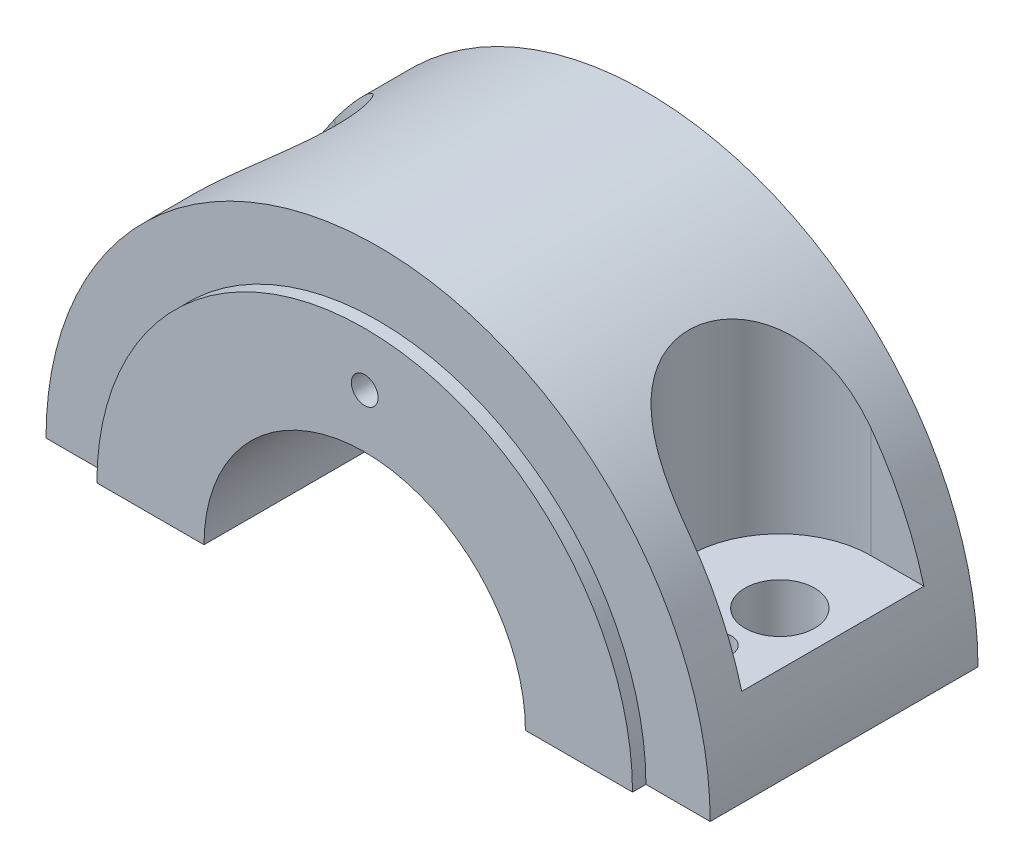
SolidWorks part; units mm, degrees
material "ZG270-500"
ref_plane "Front Plane" through (0, 0, 0) normal (0, 0, 1) x (1, 0, 0)
ref_plane "Top Plane" through (0, 0, 0) normal (0, 1, 0) x (1, 0, 0)
ref_plane "Right Plane" through (0, 0, 0) normal (1, 0, 0) x (0, 0, -1)
sketch "Sketch1" plane through (0, 0, 0) normal (0, 0, 1) x (1, 0, 0)
  line L0 (-62, 0) -> (-30, 0)
  line L1 (30, 0) -> (62, 0)
  arc A0 (62, 0) -> (-62, 0) centre (0, 0) ccw
  arc A1 (30, 0) -> (-30, 0) centre (0, 0) ccw
  dimension "D1" = 62
  dimension "D2" = 30
extrude "Boss-Extrude1" add sketch "Sketch1" along normal mid plane 50
sketch "Sketch2" plane through (0, 0, 0) normal (0, 0, 1) x (1, 0, 0)
  line L0 (-50, 0) -> (-30, 0)
  line L1 (30, 0) -> (50, 0)
  arc A0 (50, 0) -> (-50, 0) centre (0, 0) ccw
  arc A1 (30, 0) -> (-30, 0) centre (0, 0) ccw
  dimension "D1" = 50
  dimension "D2" = 30
extrude "Boss-Extrude2" add sketch "Sketch2" along normal mid plane 55
ref_plane "Plane1" through (0, 16, 0) normal (0, 1, 0) x (1, 0, 0)
sketch "Sketch3" plane through (0, 16, 0) normal (0, 1, 0) x (1, 0, 0)
  line L0 (-76.112, 0) -> (-75, 0) construction
  line L1 (0, 53.7818) -> (0, -41.5827) construction
  line L3 (-49.5568, 0) -> (74.644, 0) construction
  line L4 (-75, 17) -> (-50, 17)
  line L5 (-75, 17) -> (-75, -17)
  line L6 (-75, -17) -> (-50, -17)
  line L7 (75, -17) -> (50, -17)
  line L8 (75, 17) -> (75, -17)
  line L9 (75, 17) -> (50, 17)
  arc A0 (-50, -17) -> (-50, 17) centre (-50, 0) ccw
  arc A1 (50, -17) -> (50, 17) centre (50, 0) cw
  dimension "D1" = 17
  dimension "D2" = 100
  dimension "D3" = 34
  dimension "D4" = 150
extrude "Cut-Extrude1" cut sketch "Sketch3" along normal through all
sketch "Sketch4" plane through (0, 16, 0) normal (0, 1, 0) x (1, 0, 0)
  line L0 (-82.8581, 0) -> (79.8075, 0) construction
  line L1 (0, 63.3282) -> (0, -50.424) construction
  line L2 (-50, 68.9624) -> (-50, -54.7975) construction
  line L3 (50, 68.9624) -> (50, -54.7975) construction
  circle A0 centre (-50, 0) radius 6.5
  circle A1 centre (-50, 12) radius 3
  circle A2 centre (50, 0) radius 6.5
  circle A3 centre (50, -12) radius 3
  dimension "D4" = 6
  dimension "D5" = 13
  dimension "D1" = 100
  dimension "D2" = 12
  dimension "D3" = 12
extrude "Cut-Extrude2" cut sketch "Sketch4" against normal through all
hole_wizard "M6 Tapped Hole1" positions "Sketch6" profile "Sketch5" tap size "M6" standard "GB"
sketch "Sketch6" plane through (0, 0, 27.5) normal (0, 0, 1) x (1, 0, 0)
  line L0 (0, -69.576) -> (0, 86.8142) construction
  circle A0 centre (0, 0) radius 40 construction
  point P0 (0, 40)
  dimension "D1" = 80
sketch "Sketch5" plane through (0, 40, 27.5) normal (1, 0, 0) x (0, -1, 0)
  line L0 (0, 0) -> (0, 18.5022)
  line L1 (0, 18.5022) -> (2.5, 17)
  line L2 (2.5, 17) -> (2.5, 0)
  line L5 (2.5, 0) -> (0, 0)
  line L10 (0, 18.5022) -> (-2.5, 17) construction
  line L11 (0, -6.35) -> (0, 107.95) construction
  dimension "螺纹孔钻头直径" = 5
  dimension "螺纹孔钻头深度" = 17
  dimension "导头角度" = 118
cosmetic thread "Cosmetic Thread1" parameters "D1"=12, "D2"=6
